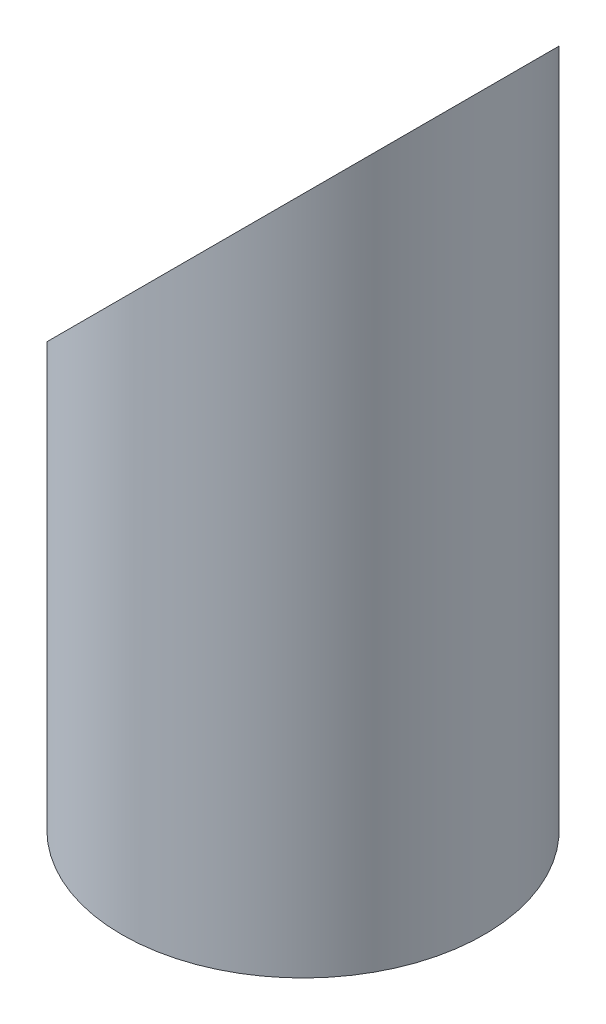
from build123d import *

# Parameters (mm, degrees)
SKETCH1_R               = 19.05
SKETCH1_R_2             = 17.05
BOSS_EXTRUDE1_DEPTH     = 77
CUT_EXTRUDE1_DEPTH      = 82.576988177
CUT_EXTRUDE1_DEPTH_BACK = 82.576988177


with BuildPart() as part:
    # Sketch1 → Boss-Extrude1 (new body)
    with BuildSketch(Plane(origin=(0, 0, 0), x_dir=(1, 0, 0), z_dir=(0, 1, 0))):
        with Locations(Location((0, 0, 0), (0, 0, 270))):
            Circle(SKETCH1_R)
        with Locations(Location((0, 0, 0), (0, 0, 270))):
            Circle(SKETCH1_R_2, mode=Mode.SUBTRACT)
    extrude(amount=BOSS_EXTRUDE1_DEPTH)

    # Sketch2 → Cut-Extrude1 (cut, two sides: drawn at the far end of the back side and taken through both)
    with BuildSketch(Plane.XY.offset(-CUT_EXTRUDE1_DEPTH_BACK)):
        Polygon((19.05, 77), (-19.05, 38.9), (-19.05, 77), align=None)
    extrude(amount=CUT_EXTRUDE1_DEPTH + CUT_EXTRUDE1_DEPTH_BACK, mode=Mode.SUBTRACT)


solid = part.part
